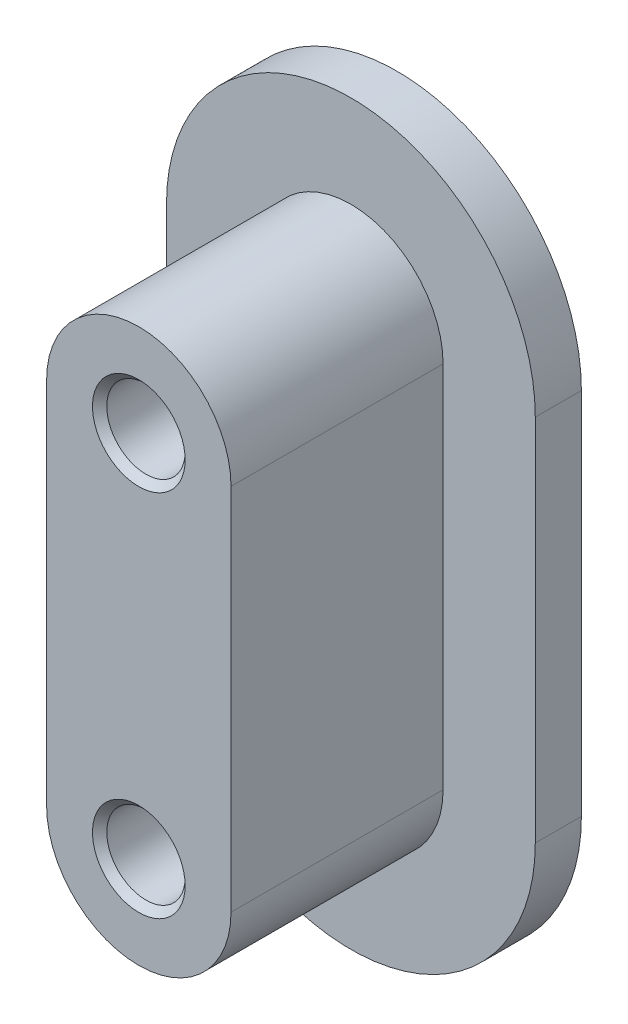
SolidWorks part; units mm, degrees
ref_plane "前视基准面" through (0, 0, 0) normal (0, 0, 1) x (1, 0, 0)
ref_plane "上视基准面" through (0, 0, 0) normal (0, 1, 0) x (1, 0, 0)
ref_plane "右视基准面" through (0, 0, 0) normal (1, 0, 0) x (0, 0, -1)
sketch "草图1" plane through (0, 0, 0) normal (0, 0, 1) x (1, 0, 0)
  line L0 (-70, -60) -> (-70, -100) construction
  line L1 (-60, -60) -> (-60, -100)
  line L2 (-80, -60) -> (-80, -100)
  line L3 (80, -125) -> (-80, -125) construction
  line L4 (-100, -105) -> (-100, 105) construction
  arc A0 (-60, -60) -> (-80, -60) centre (-70, -60) ccw
  arc A1 (-80, -100) -> (-60, -100) centre (-70, -100) ccw
  point P2 (-70, -80)
  point P7 (-67.5577, -59.673)
  dimension "D1" = 10
  dimension "D2" = 40
  dimension "D3" = 25
  dimension "D4" = 20
extrude "凸台-拉伸1" add sketch "草图1" along normal blind 28
sketch "草图2" plane through (0, 0, 0) normal (0, 0, 1) x (1, 0, 0)
  line L4 (-90, -60) -> (-90, -100)
  line L5 (-50, -100) -> (-50, -60)
  line L6 (-90, -60) -> (-90, -100)
  line L7 (-50, -100) -> (-50, -60)
  arc A4 (-50, -60) -> (-90, -60) centre (-70, -60) ccw
  arc A5 (-90, -100) -> (-50, -100) centre (-70, -100) ccw
  arc A6 (-50, -60) -> (-90, -60) centre (-70, -60) ccw
  arc A7 (-90, -100) -> (-50, -100) centre (-70, -100) ccw
  dimension "D1" = 10
extrude "凸台-拉伸2" add sketch "草图2" along normal blind 5
hole_wizard "M10 螺纹孔1" positions "草图4" profile "草图5" tap size "M10" standard "GB"
sketch "草图4" plane through (0, 0, 28) normal (0, 0, 1) x (1, 0, 0)
  point P0 (-70, -60)
  point P3 (-70, -100)
sketch "草图5" plane through (-70, -60, 28) normal (1, 0, 0) x (0, -1, 0)
  line L0 (0, 0) -> (0, 24.5)
  line L1 (0, 24.5) -> (4.25, 21.9463)
  line L2 (4.25, 21.9463) -> (4.25, 0.775)
  line L3 (4.25, 0.775) -> (5.025, 0)
  line L5 (5.025, 0) -> (0, 0)
  line L6 (-4.25, 0.775) -> (-5.025, 0) construction
  line L10 (0, 24.5) -> (-4.25, 21.9463) construction
  line L11 (0, -6.35) -> (0, 107.95) construction
  dimension "螺纹孔钻头直径" = 8.5
  dimension "螺纹孔钻头深度" = 24.5
  dimension "近端锥形沉头孔直径" = 10.05
  dimension "近端锥形沉头孔角度" = 90
  dimension "导头角度" = 118
cosmetic thread "孔螺蚊线1" parameters "D1"=20, "D2"=10
cosmetic thread "孔螺蚊线2" parameters "D1"=20, "D2"=10
